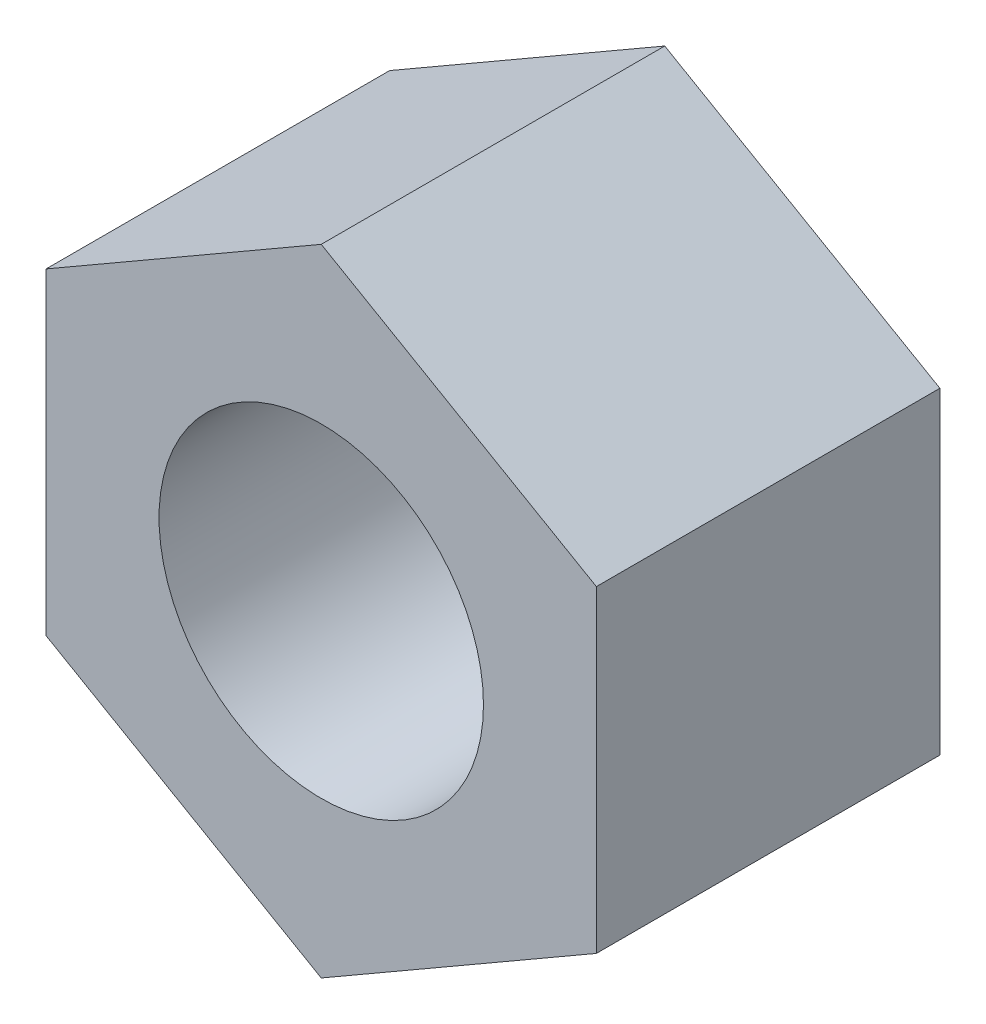
from build123d import *

# Parameters (mm, degrees)
BOSS_EXTRUDE1_DEPTH = 5.4
M12_TAPPED_HOLE1_D  = 10.2


with BuildPart() as part:
    # Sketch1 → Boss-Extrude1 (new, symmetric)
    with BuildSketch(Plane.XY):
        Polygon((8.65, -4.994079828), (8.65, 4.994079828), (0, 9.988159657), (-8.65, 4.994079828), (-8.65, -4.994079828), (0, -9.988159657), align=None)
    extrude(amount=BOSS_EXTRUDE1_DEPTH, both=True)

    # M12 Tapped Hole1 (through all)
    with Locations(Plane.XY.offset(5.4)):
        with Locations((0, 0)):
            Hole(M12_TAPPED_HOLE1_D / 2)


solid = part.part
